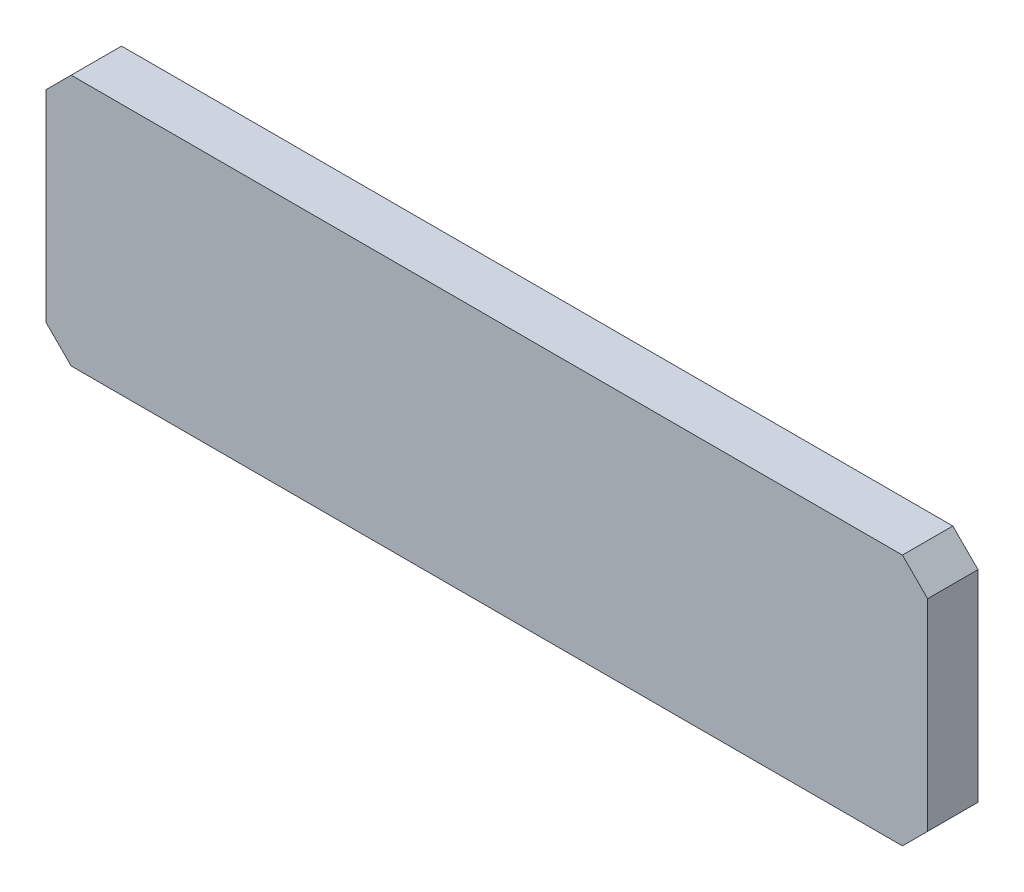
SolidWorks part; units mm, degrees
material "Q345"
ref_plane "前视基准面" through (0, 0, 0) normal (0, 0, 1) x (1, 0, 0)
ref_plane "上视基准面" through (0, 0, 0) normal (0, 1, 0) x (1, 0, 0)
ref_plane "右视基准面" through (0, 0, 0) normal (1, 0, 0) x (0, 0, -1)
sketch "草图1" plane through (0, 0, 0) normal (0, 0, 1) x (1, 0, 0)
  line L1 (-350, 100) -> (350, 100)
  line L2 (-350, 100) -> (-350, -100)
  line L3 (-350, -100) -> (350, -100)
  line L4 (350, 100) -> (350, -100)
  line L5 (-350, 100) -> (350, -100) construction
  line L6 (-350, -100) -> (350, 100) construction
  point P0 (0, 0)
  dimension "D1" = 700
  dimension "D2" = 200
extrude "凸台-拉伸1" add sketch "草图1" along normal blind 40
chamfer "倒角1" distance 20 angle 45 4 edges at (350, -100, 20) (350, 100, 20) (-350, -100, 20) (-350, 100, 20)
sketch "草图2" plane through (0, 0, 40) normal (0, 0, 1) x (1, 0, 0)
  line L0 (-350, 0) -> (350, 0) construction
  line L1 (-350, 80) -> (-350, -80) construction
  line L2 (350, -80) -> (350, 80) construction
  line L3 (300, -60) -> (-200, -60) construction
  line L4 (300, 60) -> (-200, 60) construction
  circle A0 centre (300, -60) radius 16
  circle A1 centre (200, -60) radius 16
  circle A2 centre (120, -60) radius 16
  circle A3 centre (40, -60) radius 16
  circle A4 centre (-200, -60) radius 16
  circle A5 centre (-200, 60) radius 16
  circle A6 centre (40, 60) radius 16
  circle A7 centre (120, 60) radius 16
  circle A8 centre (200, 60) radius 16
  circle A9 centre (300, 60) radius 16
  dimension "D1" = 32
  dimension "D2" = 100
  dimension "D3" = 50
  dimension "D4" = 80
  dimension "D5" = 80
  dimension "D6" = 240
  dimension "D7" = 120
